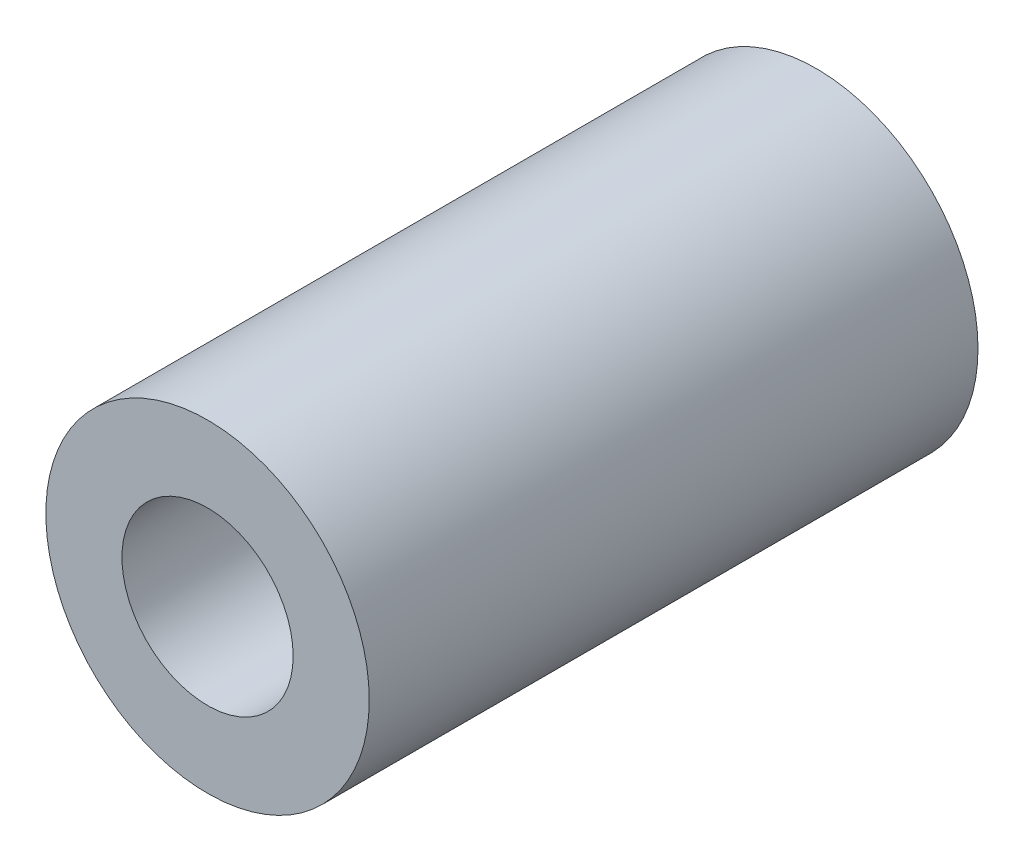
from build123d import *

# Parameters (mm, degrees)
SKETCH1_R           = 8.5
SKETCH1_R_2         = 4.5
BOSS_EXTRUDE1_DEPTH = 32


with BuildPart() as part:
    # Sketch1 → Boss-Extrude1 (new body)
    with BuildSketch(Plane.XY):
        Circle(SKETCH1_R)
        Circle(SKETCH1_R_2, mode=Mode.SUBTRACT)
    extrude(amount=BOSS_EXTRUDE1_DEPTH)


solid = part.part
